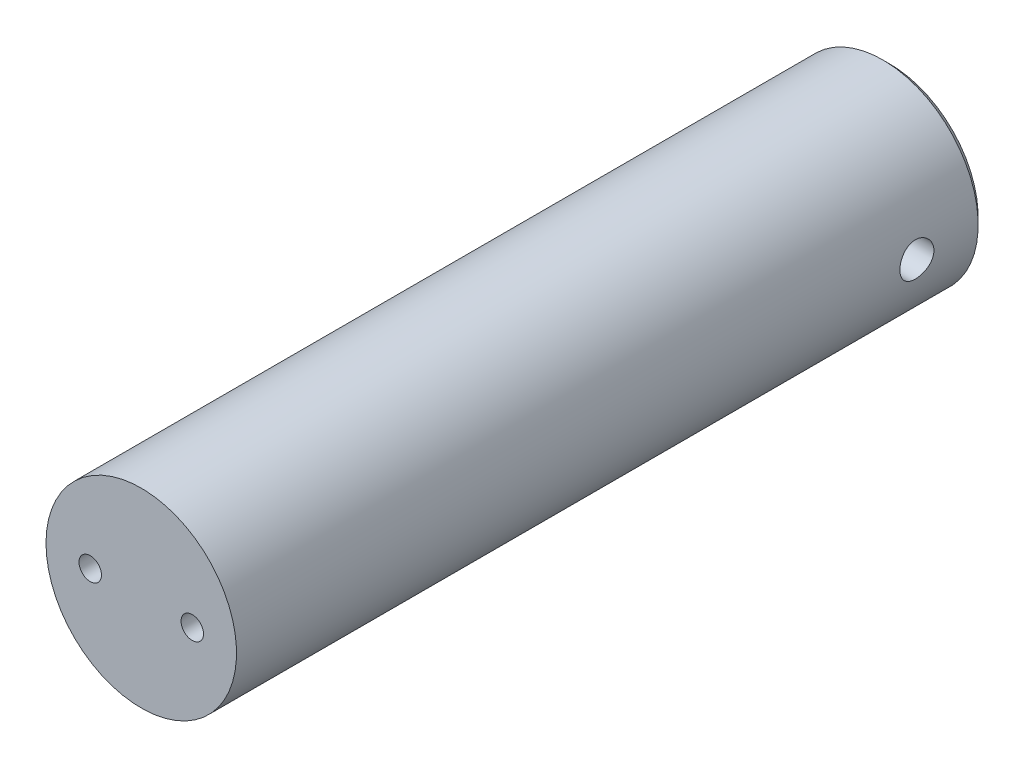
SolidWorks part; units mm, degrees
material "304"
ref_plane "Front Plane" through (0, 0, 0) normal (0, 0, 1) x (1, 0, 0)
ref_plane "Top Plane" through (0, 0, 0) normal (0, 1, 0) x (1, 0, 0)
ref_plane "Right Plane" through (0, 0, 0) normal (1, 0, 0) x (0, 0, -1)
sketch "Sketch1" plane through (0, 0, 0) normal (0, 1, 0) x (1, 0, 0)
  line L0 (-9.05, 110) -> (-14, 110)
  line L1 (-14, 110) -> (-14, 0)
  line L2 (-14, 0) -> (0, 0)
  line L3 (-9.05, 110) -> (-9.05, 50)
  line L4 (-9.05, 50) -> (0, 50)
  line L5 (0, 50) -> (0, 0)
  dimension "D1" = 14
  dimension "D2" = 9.05
  dimension "D3" = 110
  dimension "D4" = 60
revolve "Revolve1" add sketch "Sketch1" angle 360 about L5
sketch "Sketch2" plane through (0, 0, 0) normal (0, 0, 1) x (1, 0, 0)
  point P0 (-7.5, 0)
  point P1 (7.5, 0)
  dimension "D1" = 15
  dimension "D2" = 7.5
hole_wizard "M4 Tapped Hole1" positions "3DSketch1" profile "Sketch3" tap size "M4" standard "GB"
sketch3d "3DSketch1"
  point P0 (-7.5, 0, 0)
  point P3 (7.5, 0, 0)
sketch "Sketch3" plane through (-7.5, 0, 0) normal (1, 0, 0) x (0, -1, 0)
  line L0 (0, 0) -> (0, 11.0914)
  line L1 (0, 11.0914) -> (1.65, 10.1)
  line L2 (1.65, 10.1) -> (1.65, 0)
  line L5 (1.65, 0) -> (0, 0)
  line L10 (0, 11.0914) -> (-1.65, 10.1) construction
  line L11 (0, -6.35) -> (0, 107.95) construction
  dimension "螺纹孔钻头直径" = 3.3
  dimension "螺纹孔钻头深度" = 10.1
  dimension "导头角度" = 118
cosmetic thread "Cosmetic Thread3" parameters "D1"=8, "D2"=4
cosmetic thread "Cosmetic Thread4" parameters "D1"=8, "D2"=4
ref_plane "Plane1" through (14, 0, 0) normal (1, 0, 0) x (0, 0, -1)
sketch "Sketch4" plane through (14, 0, 0) normal (1, 0, 0) x (0, 0, -1)
  line L0 (110, 0) -> (100, 0) construction
  line L1 (110, -14) -> (110, 14) construction
  dimension "D1" = 10
hole_wizard "M6 Tapped Hole1" positions "3DSketch2" profile "Sketch5" tap size "M6" standard "GB"
sketch3d "3DSketch2"
  point P0 (14, 0, -100)
sketch "Sketch5" plane through (14, 0, -100) normal (0, 1, 0) x (0, 0, -1)
  line L0 (0, 0) -> (0, 18.5022)
  line L1 (0, 18.5022) -> (2.5, 17)
  line L2 (2.5, 17) -> (2.5, 0)
  line L5 (2.5, 0) -> (0, 0)
  line L10 (0, 18.5022) -> (-2.5, 17) construction
  line L11 (0, -6.35) -> (0, 107.95) construction
  dimension "螺纹孔钻头直径" = 5
  dimension "螺纹孔钻头深度" = 17
  dimension "导头角度" = 118
cosmetic thread "Cosmetic Thread5" parameters "D1"=5.3022, "D2"=6
chamfer "Chamfer1" distance 1 angle 45 2 edges at (-14, 0, -110) (-9.05, 0, -110)
